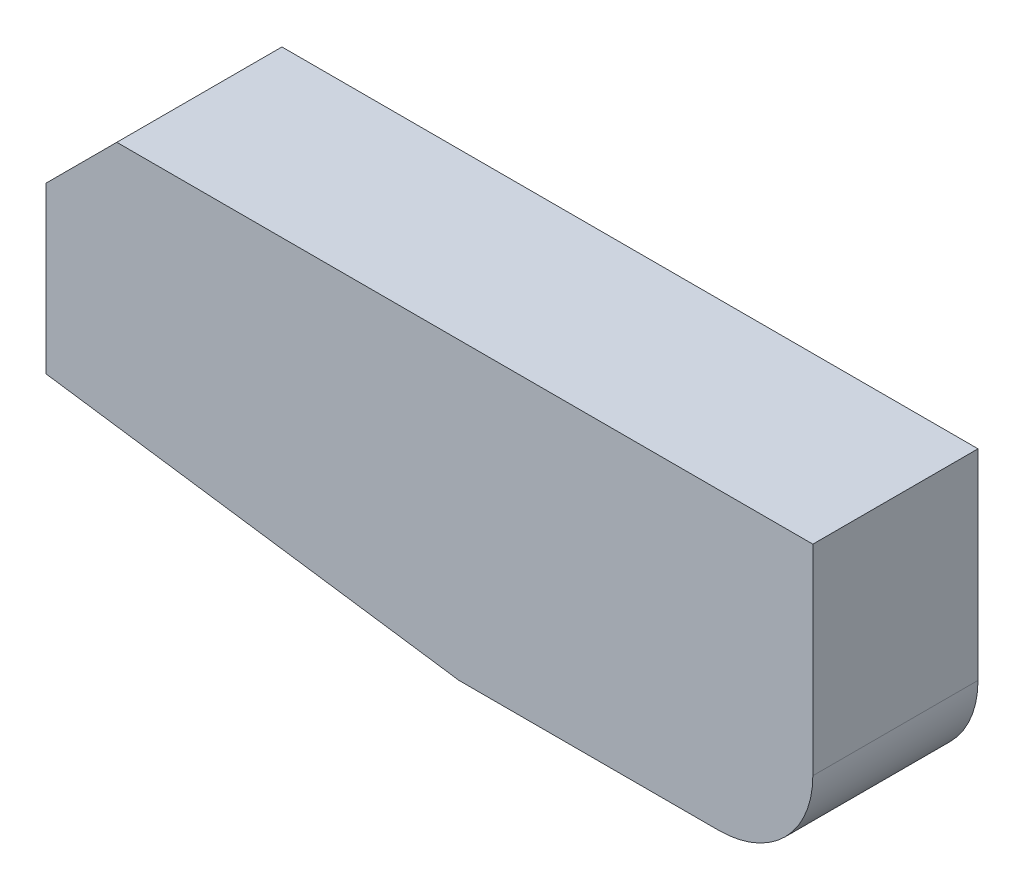
from build123d import *

# Parameters (mm, degrees)
EXTRUDE_1_DEPTH = 7
CHAMFER_1_SIZE  = 6
FILLET_1_R      = 8


with BuildPart() as part:
    # 草图1 → 凸台-拉伸1 (new, symmetric)
    with BuildSketch(Plane.XY):
        Polygon((0, 5), (0, 25), (65, 25), (65, 0), (35, 0), align=None)
    extrude(amount=EXTRUDE_1_DEPTH, both=True)

    # 倒角1
    chamfer_1_edges = [part.edges().sort_by_distance(p)[0] for p in [
        (0, 25, 0),
    ]]
    chamfer(chamfer_1_edges, length=CHAMFER_1_SIZE)

    # 圆角1
    fillet_1_edges = [part.edges().sort_by_distance(p)[0] for p in [
        (65, 0, 0),
    ]]
    fillet(fillet_1_edges, radius=FILLET_1_R)


solid = part.part
